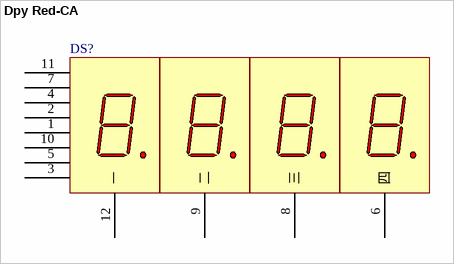
[diagram p0: symbol Dpy Red-CA]
# Altium schematic symbol library MISC89340-20.SchLib: 1 symbol
Pins are listed as number, name and electrical type; pins without a type are passive.


## Dpy Red-CA
designator DS?
7.62 mm Black Surface HER 7-Segment Display: CA, RH DP
footprint 四位数码管
pins: 1, 2, 3, 4, 5, 6 四, 7, 8 三, 9 二, 10, 11, 12 一